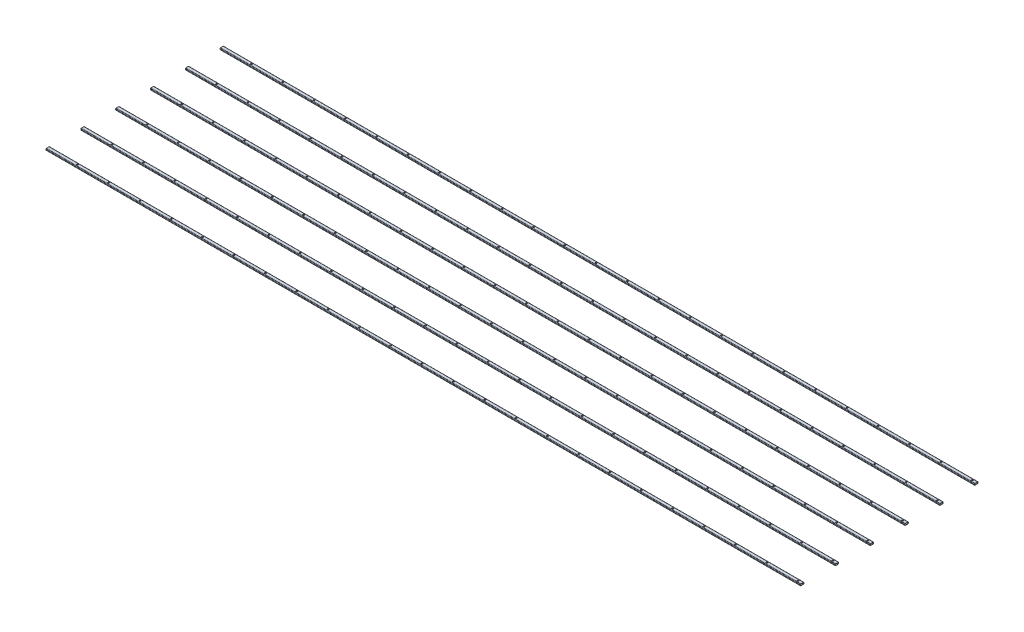
from build123d import *

# Parameters (mm, degrees)
GB_6728_1986_RECTANGULAR_HOLLOW_SECTION_DEPTH = 6500
GB_6728_1986_RECTANGULAR_HOLLOW_SECT_2_DEPTH  = 6500
GB_6728_1986_RECTANGULAR_HOLLOW_SECT_3_DEPTH  = 6500
GB_6728_1986_RECTANGULAR_HOLLOW_SECT_4_DEPTH  = 6500
GB_6728_1986_RECTANGULAR_HOLLOW_SECT_5_DEPTH  = 6500
GB_6728_1986_RECTANGULAR_HOLLOW_SECT_6_DEPTH  = 6500
SKETCH6_R                                     = 6.5
CUT_EXTRUDE1_DEPTH                            = 6675.237784197
LPATTERN2_COUNT                               = 6
LPATTERN2_PITCH                               = 300
LPATTERN2_COUNT_DIR2                          = 24
LPATTERN2_PITCH_DIR2                          = 270


with BuildPart() as part:
    # Sketch17 → Gb/6728-1986 rectangular hollow section 030 X 20 X 2 (new body)
    with BuildSketch(Plane(origin=(0, 0, -1500), x_dir=(0, -1, 0), z_dir=(1, 0, 0))):
        with BuildLine():
            Line((-3.5, -15), (3.5, -15))
            ThreePointArc((3.5, -15), (6.328427125, -13.828427125), (7.5, -11))
            Line((7.5, -11), (7.5, 11))
            ThreePointArc((7.5, 11), (6.328427125, 13.828427125), (3.5, 15))
            Line((3.5, 15), (-3.5, 15))
            ThreePointArc((-3.5, 15), (-6.328427125, 13.828427125), (-7.5, 11))
            Line((-7.5, 11), (-7.5, -11))
            ThreePointArc((-7.5, -11), (-6.328427125, -13.828427125), (-3.5, -15))
        make_face()
        with BuildLine():
            Line((-3.5, -13), (3.5, -13))
            ThreePointArc((3.5, -13), (4.914213562, -12.414213562), (5.5, -11))
            Line((5.5, -11), (5.5, 11))
            ThreePointArc((5.5, 11), (4.914213562, 12.414213562), (3.5, 13))
            Line((3.5, 13), (-3.5, 13))
            ThreePointArc((-3.5, 13), (-4.914213562, 12.414213562), (-5.5, 11))
            Line((-5.5, 11), (-5.5, -11))
            ThreePointArc((-5.5, -11), (-4.914213562, -12.414213562), (-3.5, -13))
        make_face(mode=Mode.SUBTRACT)
    extrude(amount=GB_6728_1986_RECTANGULAR_HOLLOW_SECTION_DEPTH)

    # Sketch6 → Cut-Extrude1 (cut, through all)
    with BuildSketch(Plane(origin=(0, 7.5, 0), x_dir=(1, 0, 0), z_dir=(0, 1, 0))):
        with Locations(Location((6465, 1500, 0), (0, 0, 270))):
            Circle(SKETCH6_R)
    cut_extrude1 = extrude(amount=-CUT_EXTRUDE1_DEPTH, mode=Mode.SUBTRACT)


with BuildPart() as body_2:
    # Sketch17 on segment 2 (carried to segment 2) → Gb_6728-1986 rectangular hollow sect 2 (new body)
    with BuildSketch(Plane(origin=(0, 0, -1200), x_dir=(0, -1, 0), z_dir=(1, 0, 0))):
        with BuildLine():
            Line((-3.5, -15), (3.5, -15))
            ThreePointArc((3.5, -15), (6.328427125, -13.828427125), (7.5, -11))
            Line((7.5, -11), (7.5, 11))
            ThreePointArc((7.5, 11), (6.328427125, 13.828427125), (3.5, 15))
            Line((3.5, 15), (-3.5, 15))
            ThreePointArc((-3.5, 15), (-6.328427125, 13.828427125), (-7.5, 11))
            Line((-7.5, 11), (-7.5, -11))
            ThreePointArc((-7.5, -11), (-6.328427125, -13.828427125), (-3.5, -15))
        make_face()
        with BuildLine():
            Line((-3.5, -13), (3.5, -13))
            ThreePointArc((3.5, -13), (4.914213562, -12.414213562), (5.5, -11))
            Line((5.5, -11), (5.5, 11))
            ThreePointArc((5.5, 11), (4.914213562, 12.414213562), (3.5, 13))
            Line((3.5, 13), (-3.5, 13))
            ThreePointArc((-3.5, 13), (-4.914213562, 12.414213562), (-5.5, 11))
            Line((-5.5, 11), (-5.5, -11))
            ThreePointArc((-5.5, -11), (-4.914213562, -12.414213562), (-3.5, -13))
        make_face(mode=Mode.SUBTRACT)
    extrude(amount=GB_6728_1986_RECTANGULAR_HOLLOW_SECT_2_DEPTH)


with BuildPart() as body_3:
    # Sketch17 on segment 3 (carried to segment 3) → Gb_6728-1986 rectangular hollow sect 3 (new body)
    with BuildSketch(Plane(origin=(0, 0, -900), x_dir=(0, -1, 0), z_dir=(1, 0, 0))):
        with BuildLine():
            Line((-3.5, -15), (3.5, -15))
            ThreePointArc((3.5, -15), (6.328427125, -13.828427125), (7.5, -11))
            Line((7.5, -11), (7.5, 11))
            ThreePointArc((7.5, 11), (6.328427125, 13.828427125), (3.5, 15))
            Line((3.5, 15), (-3.5, 15))
            ThreePointArc((-3.5, 15), (-6.328427125, 13.828427125), (-7.5, 11))
            Line((-7.5, 11), (-7.5, -11))
            ThreePointArc((-7.5, -11), (-6.328427125, -13.828427125), (-3.5, -15))
        make_face()
        with BuildLine():
            Line((-3.5, -13), (3.5, -13))
            ThreePointArc((3.5, -13), (4.914213562, -12.414213562), (5.5, -11))
            Line((5.5, -11), (5.5, 11))
            ThreePointArc((5.5, 11), (4.914213562, 12.414213562), (3.5, 13))
            Line((3.5, 13), (-3.5, 13))
            ThreePointArc((-3.5, 13), (-4.914213562, 12.414213562), (-5.5, 11))
            Line((-5.5, 11), (-5.5, -11))
            ThreePointArc((-5.5, -11), (-4.914213562, -12.414213562), (-3.5, -13))
        make_face(mode=Mode.SUBTRACT)
    extrude(amount=GB_6728_1986_RECTANGULAR_HOLLOW_SECT_3_DEPTH)


with BuildPart() as body_4:
    # Sketch17 on segment 4 (carried to segment 4) → Gb_6728-1986 rectangular hollow sect 4 (new body)
    with BuildSketch(Plane(origin=(0, 0, 0), x_dir=(0, -1, 0), z_dir=(1, 0, 0))):
        with BuildLine():
            Line((-3.5, -15), (3.5, -15))
            ThreePointArc((3.5, -15), (6.328427125, -13.828427125), (7.5, -11))
            Line((7.5, -11), (7.5, 11))
            ThreePointArc((7.5, 11), (6.328427125, 13.828427125), (3.5, 15))
            Line((3.5, 15), (-3.5, 15))
            ThreePointArc((-3.5, 15), (-6.328427125, 13.828427125), (-7.5, 11))
            Line((-7.5, 11), (-7.5, -11))
            ThreePointArc((-7.5, -11), (-6.328427125, -13.828427125), (-3.5, -15))
        make_face()
        with BuildLine():
            Line((-3.5, -13), (3.5, -13))
            ThreePointArc((3.5, -13), (4.914213562, -12.414213562), (5.5, -11))
            Line((5.5, -11), (5.5, 11))
            ThreePointArc((5.5, 11), (4.914213562, 12.414213562), (3.5, 13))
            Line((3.5, 13), (-3.5, 13))
            ThreePointArc((-3.5, 13), (-4.914213562, 12.414213562), (-5.5, 11))
            Line((-5.5, 11), (-5.5, -11))
            ThreePointArc((-5.5, -11), (-4.914213562, -12.414213562), (-3.5, -13))
        make_face(mode=Mode.SUBTRACT)
    extrude(amount=GB_6728_1986_RECTANGULAR_HOLLOW_SECT_4_DEPTH)


with BuildPart() as body_5:
    # Sketch17 on segment 5 (carried to segment 5) → Gb_6728-1986 rectangular hollow sect 5 (new body)
    with BuildSketch(Plane(origin=(0, 0, -600), x_dir=(0, -1, 0), z_dir=(1, 0, 0))):
        with BuildLine():
            Line((-3.5, -15), (3.5, -15))
            ThreePointArc((3.5, -15), (6.328427125, -13.828427125), (7.5, -11))
            Line((7.5, -11), (7.5, 11))
            ThreePointArc((7.5, 11), (6.328427125, 13.828427125), (3.5, 15))
            Line((3.5, 15), (-3.5, 15))
            ThreePointArc((-3.5, 15), (-6.328427125, 13.828427125), (-7.5, 11))
            Line((-7.5, 11), (-7.5, -11))
            ThreePointArc((-7.5, -11), (-6.328427125, -13.828427125), (-3.5, -15))
        make_face()
        with BuildLine():
            Line((-3.5, -13), (3.5, -13))
            ThreePointArc((3.5, -13), (4.914213562, -12.414213562), (5.5, -11))
            Line((5.5, -11), (5.5, 11))
            ThreePointArc((5.5, 11), (4.914213562, 12.414213562), (3.5, 13))
            Line((3.5, 13), (-3.5, 13))
            ThreePointArc((-3.5, 13), (-4.914213562, 12.414213562), (-5.5, 11))
            Line((-5.5, 11), (-5.5, -11))
            ThreePointArc((-5.5, -11), (-4.914213562, -12.414213562), (-3.5, -13))
        make_face(mode=Mode.SUBTRACT)
    extrude(amount=GB_6728_1986_RECTANGULAR_HOLLOW_SECT_5_DEPTH)


with BuildPart() as body_6:
    # Sketch17 on segment 6 (carried to segment 6) → Gb_6728-1986 rectangular hollow sect 6 (new body)
    with BuildSketch(Plane(origin=(0, 0, -300), x_dir=(0, -1, 0), z_dir=(1, 0, 0))):
        with BuildLine():
            Line((-3.5, -15), (3.5, -15))
            ThreePointArc((3.5, -15), (6.328427125, -13.828427125), (7.5, -11))
            Line((7.5, -11), (7.5, 11))
            ThreePointArc((7.5, 11), (6.328427125, 13.828427125), (3.5, 15))
            Line((3.5, 15), (-3.5, 15))
            ThreePointArc((-3.5, 15), (-6.328427125, 13.828427125), (-7.5, 11))
            Line((-7.5, 11), (-7.5, -11))
            ThreePointArc((-7.5, -11), (-6.328427125, -13.828427125), (-3.5, -15))
        make_face()
        with BuildLine():
            Line((-3.5, -13), (3.5, -13))
            ThreePointArc((3.5, -13), (4.914213562, -12.414213562), (5.5, -11))
            Line((5.5, -11), (5.5, 11))
            ThreePointArc((5.5, 11), (4.914213562, 12.414213562), (3.5, 13))
            Line((3.5, 13), (-3.5, 13))
            ThreePointArc((-3.5, 13), (-4.914213562, 12.414213562), (-5.5, 11))
            Line((-5.5, 11), (-5.5, -11))
            ThreePointArc((-5.5, -11), (-4.914213562, -12.414213562), (-3.5, -13))
        make_face(mode=Mode.SUBTRACT)
    extrude(amount=GB_6728_1986_RECTANGULAR_HOLLOW_SECT_6_DEPTH)


with BuildPart() as lpattern2_tool:
    # LPattern2: Cut-Extrude1 6 × 24
    with Locations(*[(-j * LPATTERN2_PITCH_DIR2, 0, i * LPATTERN2_PITCH) for i in range(LPATTERN2_COUNT) for j in range(LPATTERN2_COUNT_DIR2) if (i, j) != (0, 0)]):
        add(cut_extrude1)


with BuildPart() as part_1:
    add(part.part)

    # LPattern2: cut by lpattern2_tool
    add(lpattern2_tool.part, mode=Mode.SUBTRACT)


with BuildPart() as body_2_1:
    add(body_2.part)

    # LPattern2: cut by lpattern2_tool
    add(lpattern2_tool.part, mode=Mode.SUBTRACT)


with BuildPart() as body_3_1:
    add(body_3.part)

    # LPattern2: cut by lpattern2_tool
    add(lpattern2_tool.part, mode=Mode.SUBTRACT)


with BuildPart() as body_4_1:
    add(body_4.part)

    # LPattern2: cut by lpattern2_tool
    add(lpattern2_tool.part, mode=Mode.SUBTRACT)


with BuildPart() as body_5_1:
    add(body_5.part)

    # LPattern2: cut by lpattern2_tool
    add(lpattern2_tool.part, mode=Mode.SUBTRACT)


with BuildPart() as body_6_1:
    add(body_6.part)

    # LPattern2: cut by lpattern2_tool
    add(lpattern2_tool.part, mode=Mode.SUBTRACT)


solid = Compound([part_1.part, body_2_1.part, body_3_1.part, body_4_1.part, body_5_1.part, body_6_1.part])
